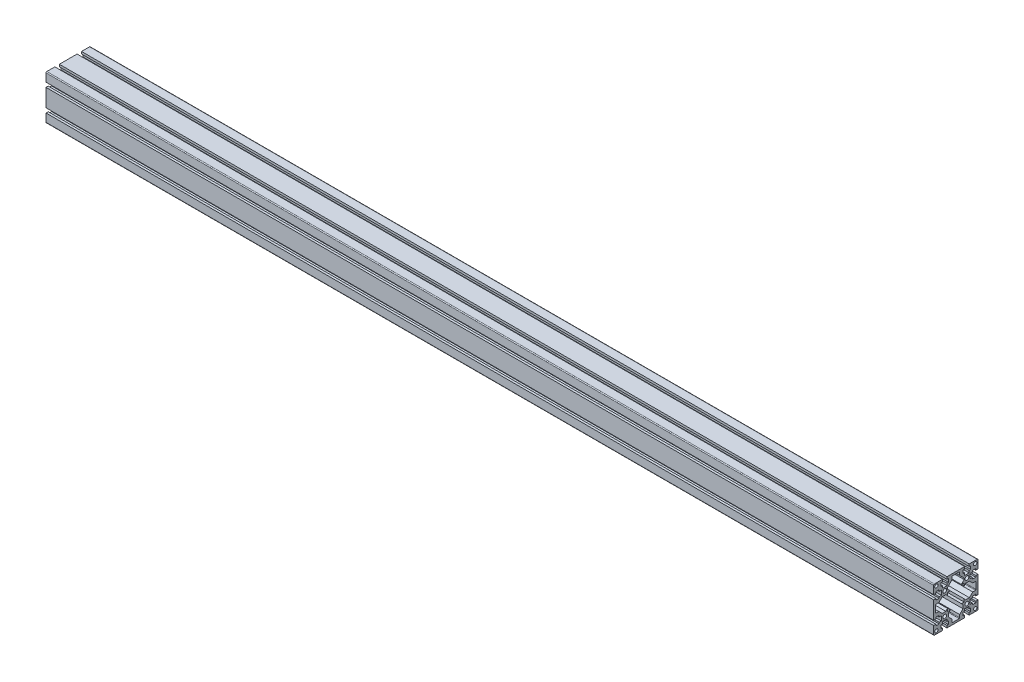
from build123d import *

# Parameters (mm, degrees)
SKETCH1_R                                 = 3.4
SKETCH1_R_2                               = 3
ALUMINIUM_PROFILE_80_X_80G_X_R1_5_1_DEPTH = 1600
SKETCH10_R                                = 3
CUT_EXTRUDE1_DEPTH                        = 1601.999687695


with BuildPart() as part:
    # Sketch1 → Aluminium profile 80 X 80G X R1.5(1) (new body)
    with BuildSketch(Plane.YZ.offset(-530.344827586)):
        with BuildLine():
            Line((-24.05, 40), (-24.05, 36))
            Line((-24.05, 36), (-26.75, 36))
            Line((-26.75, 36), (-26.75, 30))
            Line((-26.75, 30), (-24.05, 30))
            Line((-24.05, 30), (-24.05, 26))
            Line((-24.05, 26), (-15.95, 26))
            Line((-15.95, 26), (-15.95, 30))
            Line((-15.95, 30), (-13.25, 30))
            Line((-13.25, 30), (-13.25, 36))
            Line((-13.25, 36), (-15.95, 36))
            Line((-15.95, 36), (-15.95, 40))
            Line((-15.95, 40), (15.95, 40))
            Line((15.95, 40), (15.95, 36))
            Line((15.95, 36), (13.25, 36))
            Line((13.25, 36), (13.25, 30))
            Line((13.25, 30), (15.95, 30))
            Line((15.95, 30), (15.95, 26))
            Line((15.95, 26), (24.05, 26))
            Line((24.05, 26), (24.05, 30))
            Line((24.05, 30), (26.75, 30))
            Line((26.75, 30), (26.75, 36))
            Line((26.75, 36), (24.05, 36))
            Line((24.05, 36), (24.05, 40))
            Line((24.05, 40), (38.5, 40))
            ThreePointArc((38.5, 40), (39.560660172, 39.560660172), (40, 38.5))
            Line((40, 38.5), (40, 24.05))
            Line((40, 24.05), (36, 24.05))
            Line((36, 24.05), (36, 26.75))
            Line((36, 26.75), (30, 26.75))
            Line((30, 26.75), (30, 24.05))
            Line((30, 24.05), (26, 24.05))
            Line((26, 24.05), (26, 15.95))
            Line((26, 15.95), (30, 15.95))
            Line((30, 15.95), (30, 13.25))
            Line((30, 13.25), (36, 13.25))
            Line((36, 13.25), (36, 15.95))
            Line((36, 15.95), (40, 15.95))
            Line((40, 15.95), (40, -15.95))
            Line((40, -15.95), (36, -15.95))
            Line((36, -15.95), (36, -13.25))
            Line((36, -13.25), (30, -13.25))
            Line((30, -13.25), (30, -15.95))
            Line((30, -15.95), (26, -15.95))
            Line((26, -15.95), (26, -24.05))
            Line((26, -24.05), (30, -24.05))
            Line((30, -24.05), (30, -26.75))
            Line((30, -26.75), (36, -26.75))
            Line((36, -26.75), (36, -24.05))
            Line((36, -24.05), (40, -24.05))
            Line((40, -24.05), (40, -38.5))
            ThreePointArc((40, -38.5), (39.560660172, -39.560660172), (38.5, -40))
            Line((38.5, -40), (24.05, -40))
            Line((24.05, -40), (24.05, -36))
            Line((24.05, -36), (26.75, -36))
            Line((26.75, -36), (26.75, -30))
            Line((26.75, -30), (24.05, -30))
            Line((24.05, -30), (24.05, -26))
            Line((24.05, -26), (15.95, -26))
            Line((15.95, -26), (15.95, -30))
            Line((15.95, -30), (13.25, -30))
            Line((13.25, -30), (13.25, -36))
            Line((13.25, -36), (15.95, -36))
            Line((15.95, -36), (15.95, -40))
            Line((15.95, -40), (-15.95, -40))
            Line((-15.95, -40), (-15.95, -36))
            Line((-15.95, -36), (-13.25, -36))
            Line((-13.25, -36), (-13.25, -30))
            Line((-13.25, -30), (-15.95, -30))
            Line((-15.95, -30), (-15.95, -26))
            Line((-15.95, -26), (-24.05, -26))
            Line((-24.05, -26), (-24.05, -30))
            Line((-24.05, -30), (-26.75, -30))
            Line((-26.75, -30), (-26.75, -36))
            Line((-26.75, -36), (-24.05, -36))
            Line((-24.05, -36), (-24.05, -40))
            Line((-24.05, -40), (-38.5, -40))
            ThreePointArc((-38.5, -40), (-39.560660172, -39.560660172), (-40, -38.5))
            Line((-40, -38.5), (-40, -24.05))
            Line((-40, -24.05), (-36, -24.05))
            Line((-36, -24.05), (-36, -26.75))
            Line((-36, -26.75), (-30, -26.75))
            Line((-30, -26.75), (-30, -24.05))
            Line((-30, -24.05), (-26, -24.05))
            Line((-26, -24.05), (-26, -15.95))
            Line((-26, -15.95), (-30, -15.95))
            Line((-30, -15.95), (-30, -13.25))
            Line((-30, -13.25), (-36, -13.25))
            Line((-36, -13.25), (-36, -15.95))
            Line((-36, -15.95), (-40, -15.95))
            Line((-40, -15.95), (-40, 15.95))
            Line((-40, 15.95), (-36, 15.95))
            Line((-36, 15.95), (-36, 13.25))
            Line((-36, 13.25), (-30, 13.25))
            Line((-30, 13.25), (-30, 15.95))
            Line((-30, 15.95), (-26, 15.95))
            Line((-26, 15.95), (-26, 24.05))
            Line((-26, 24.05), (-30, 24.05))
            Line((-30, 24.05), (-30, 26.75))
            Line((-30, 26.75), (-36, 26.75))
            Line((-36, 26.75), (-36, 24.05))
            Line((-36, 24.05), (-40, 24.05))
            Line((-40, 24.05), (-40, 38.5))
            ThreePointArc((-40, 38.5), (-39.560660172, 39.560660172), (-38.5, 40))
            Line((-38.5, 40), (-24.05, 40))
        make_face()
        with Locations((-20, 20)):
            Circle(SKETCH1_R, mode=Mode.SUBTRACT)
        with Locations((20, 20)):
            Circle(SKETCH1_R, mode=Mode.SUBTRACT)
        with Locations((20, -20)):
            Circle(SKETCH1_R, mode=Mode.SUBTRACT)
        with Locations((-20, -20)):
            Circle(SKETCH1_R, mode=Mode.SUBTRACT)
        with Locations((-35, 35)):
            Circle(SKETCH1_R_2, mode=Mode.SUBTRACT)
        with Locations((35, 35)):
            Circle(SKETCH1_R_2, mode=Mode.SUBTRACT)
        with Locations((35, -35)):
            Circle(SKETCH1_R_2, mode=Mode.SUBTRACT)
        with BuildLine():
            Line((-13, 18), (-10, 15))
            Line((-10, 15), (-15, 15))
            Line((-15, 15), (-15, 10))
            Line((-15, 10), (-18, 13))
            Line((-18, 13), (-24.5, 13))
            Line((-24.5, 13), (-30.5, 7))
            Line((-30.5, 7), (-35.5, 7))
            ThreePointArc((-35.5, 7), (-36.207106781, 6.707106781), (-36.5, 6))
            Line((-36.5, 6), (-36.5, -6))
            ThreePointArc((-36.5, -6), (-36.207106781, -6.707106781), (-35.5, -7))
            Line((-35.5, -7), (-30.5, -7))
            Line((-30.5, -7), (-24.5, -13))
            Line((-24.5, -13), (-18, -13))
            Line((-18, -13), (-15, -10))
            Line((-15, -10), (-15, -15))
            Line((-15, -15), (-10, -15))
            Line((-10, -15), (-13, -18))
            Line((-13, -18), (-13, -24.5))
            Line((-13, -24.5), (-7, -30.5))
            Line((-7, -30.5), (-7, -35.5))
            ThreePointArc((-7, -35.5), (-6.707106781, -36.207106781), (-6, -36.5))
            Line((-6, -36.5), (6, -36.5))
            ThreePointArc((6, -36.5), (6.707106781, -36.207106781), (7, -35.5))
            Line((7, -35.5), (7, -30.5))
            Line((7, -30.5), (13, -24.5))
            Line((13, -24.5), (13, -18))
            Line((13, -18), (10, -15))
            Line((10, -15), (15, -15))
            Line((15, -15), (15, -10))
            Line((15, -10), (20, -15))
            Line((20, -15), (22.5, -15))
            Line((22.5, -15), (30.5, -7))
            Line((30.5, -7), (35.5, -7))
            ThreePointArc((35.5, -7), (36.207106781, -6.707106781), (36.5, -6))
            Line((36.5, -6), (36.5, 6))
            ThreePointArc((36.5, 6), (36.207106781, 6.707106781), (35.5, 7))
            Line((35.5, 7), (30.5, 7))
            Line((30.5, 7), (22.5, 15))
            Line((22.5, 15), (20, 15))
            Line((20, 15), (15, 10))
            Line((15, 10), (15, 15))
            Line((15, 15), (10, 15))
            Line((10, 15), (13, 18))
            Line((13, 18), (13, 24.5))
            Line((13, 24.5), (7, 30.5))
            Line((7, 30.5), (7, 35.5))
            ThreePointArc((7, 35.5), (6.707106781, 36.207106781), (6, 36.5))
            Line((6, 36.5), (-6, 36.5))
            ThreePointArc((-6, 36.5), (-6.707106781, 36.207106781), (-7, 35.5))
            Line((-7, 35.5), (-7, 30.5))
            Line((-7, 30.5), (-13, 24.5))
            Line((-13, 24.5), (-13, 18))
        make_face(mode=Mode.SUBTRACT)
    extrude(amount=ALUMINIUM_PROFILE_80_X_80G_X_R1_5_1_DEPTH)

    # Sketch10 → Cut-Extrude1 (cut, through all)
    with BuildSketch(Plane(origin=(1069.655172414, 0, 0), x_dir=(0, 0, -1), z_dir=(1, 0, 0))):
        with Locations((35, -35)):
            Circle(SKETCH10_R)
    extrude(amount=-CUT_EXTRUDE1_DEPTH, mode=Mode.SUBTRACT)


solid = part.part
